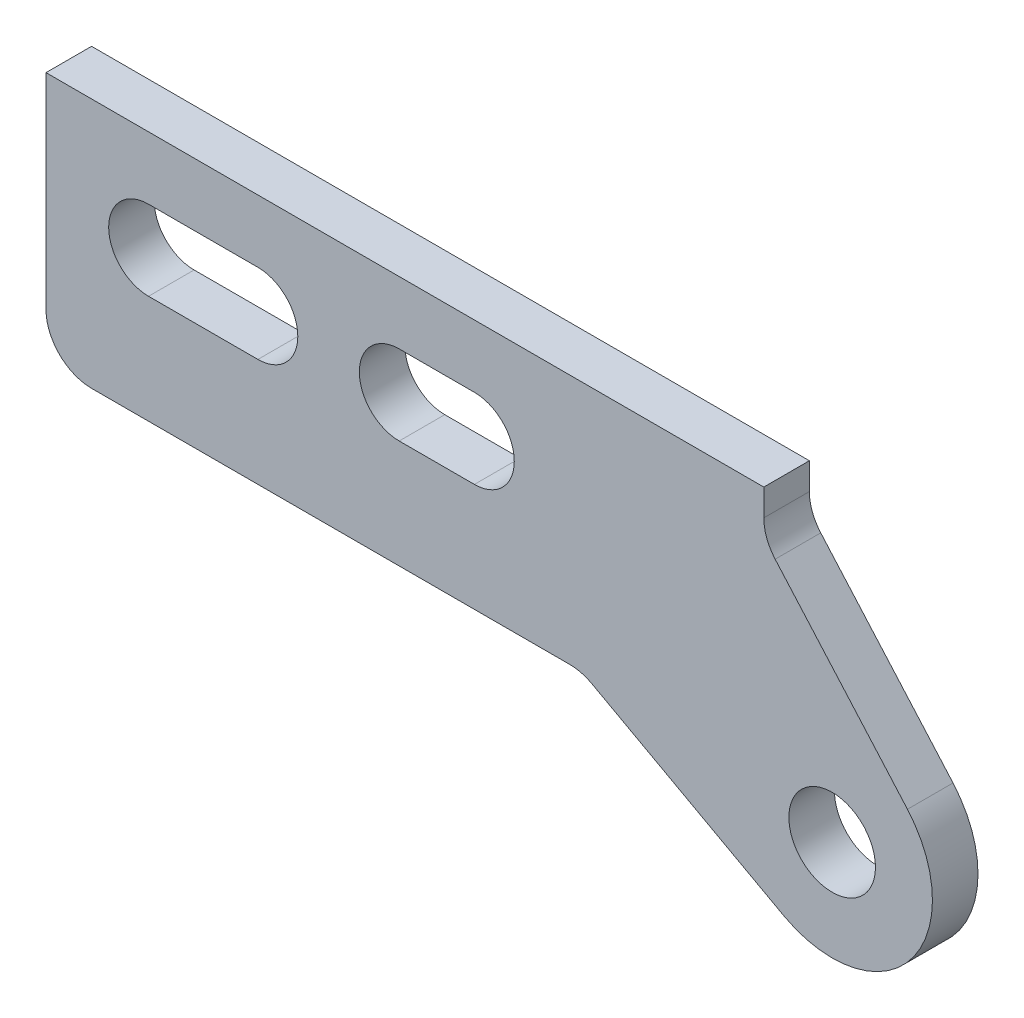
from build123d import *

# Parameters (mm, degrees)
SKETCH_3_R      = 19
EXTRUDE_2_DEPTH = 20


with BuildPart() as part:
    # 草图3 → 凸台-拉伸2 (new body)
    with BuildSketch(Plane.XY):
        with BuildLine():
            Line((0, 0), (-315, 0))
            Line((-315, 0), (-315, -90))
            ThreePointArc((-315, -90), (-309.142135624, -104.142135624), (-295, -110))
            Line((-295, -110), (-85.110940509, -110))
            ThreePointArc((-85.110940509, -110), (-80.159130316, -110.622704631), (-75.515671638, -112.452042418))
            Line((-75.515671638, -112.452042418), (8.890408484, -158.60550668))
            ThreePointArc((8.890408484, -158.60550668), (64.353360189, -147.492665271), (63.040388304, -90.942595767))
            Line((63.040388304, -90.942595767), (4.98164168, -24.925565564))
            ThreePointArc((4.98164168, -24.925565564), (1.286807242, -18.775729131), (0, -11.71765455))
            Line((0, -11.71765455), (0, 0))
        make_face()
        with Locations((30, -120)):
            Circle(SKETCH_3_R, mode=Mode.SUBTRACT)
        with BuildLine():
            Line((-270, -27.5), (-222, -27.5))
            ThreePointArc((-222, -27.5), (-204.5, -45), (-222, -62.5))
            Line((-222, -62.5), (-270, -62.5))
            ThreePointArc((-270, -62.5), (-287.5, -45), (-270, -27.5))
        make_face(mode=Mode.SUBTRACT)
        with BuildLine():
            Line((-160, -27.5), (-127, -27.5))
            ThreePointArc((-127, -27.5), (-109.5, -45), (-127, -62.5))
            Line((-127, -62.5), (-160, -62.5))
            ThreePointArc((-160, -62.5), (-177.5, -45), (-160, -27.5))
        make_face(mode=Mode.SUBTRACT)
    extrude(amount=EXTRUDE_2_DEPTH)


solid = part.part
